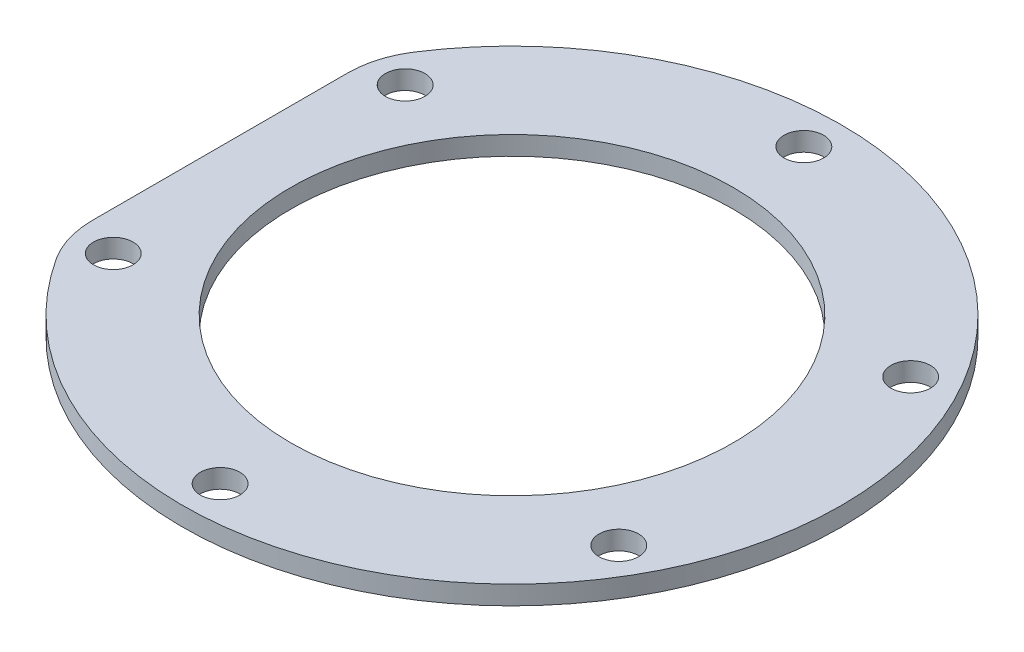
SolidWorks part; units mm, degrees
material "6061 合金"
ref_plane "前视基准面" through (0, 0, 0) normal (0, 0, 1) x (1, 0, 0)
ref_plane "上视基准面" through (0, 0, 0) normal (0, 1, 0) x (1, 0, 0)
ref_plane "右视基准面" through (0, 0, 0) normal (1, 0, 0) x (0, 0, -1)
other "Configuration Table"
sketch "草图1" plane through (0, 0, 0) normal (0, 1, 0) x (1, 0, 0)
  line L0 (-31, -13.5647) -> (-31, 13.5647)
  line L1 (-26.8468, 15.5) -> (-26.8468, -15.5) construction
  arc A0 (-29.4, -18.9905) -> (-29.4, 18.9905) centre (0, 0) ccw
  circle A1 centre (0, 0) radius 31 construction
  circle A2 centre (0, 0) radius 23.5
  circle A3 centre (0, 31) radius 2.1
  circle A4 centre (26.8468, 15.5) radius 2.1
  circle A5 centre (26.8468, -15.5) radius 2.1
  circle A6 centre (0, -31) radius 2.1
  circle A7 centre (-26.8468, -15.5) radius 2.1
  circle A8 centre (-26.8468, 15.5) radius 2.1
  arc A9 (-29.4, -18.9905) -> (-31, -13.5647) centre (-21, -13.5647) cw
  arc A10 (-31, 13.5647) -> (-29.4, 18.9905) centre (-21, 13.5647) cw
  point P20 (0, 0)
  dimension "D1" = 70
  dimension "D2" = 62
  dimension "D3" = 47
  dimension "D4" = 4.2
  dimension "D7" = 10
  dimension "D6" = 31
  dimension "D5" = 6
extrude "凸台-拉伸1" add sketch "草图1" along normal blind 2
